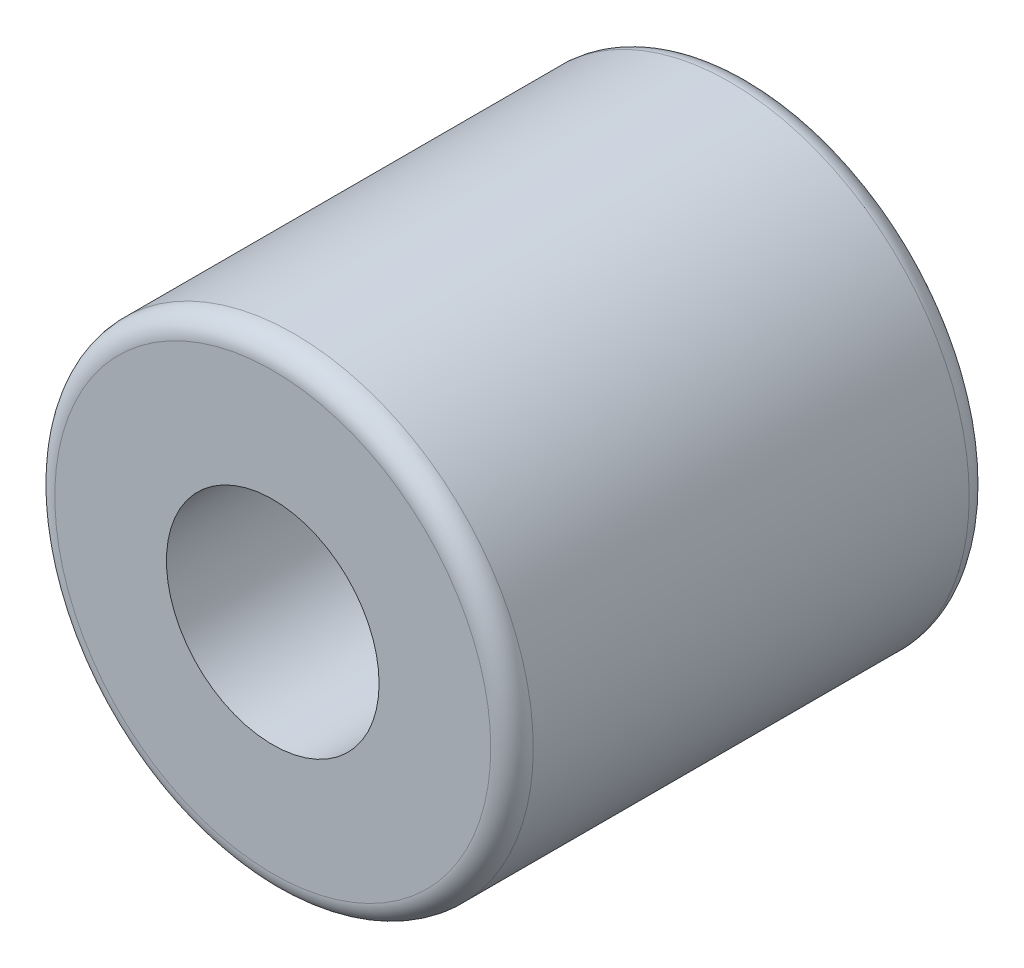
from build123d import *

# Parameters (mm, degrees)
SKETCH_1_R          = 22.5
EXTRUDE_1_DEPTH     = 45
FILLET_1_R          = 2
SKETCH_2_R          = 10
CUT_EXTRUDE_1_DEPTH = 56.113519253


with BuildPart() as part:
    # 草图1 → 凸台-拉伸1 (new body)
    with BuildSketch(Plane.XY):
        with Locations(Location((0, 0, 0), (0, 0, 180))):
            Circle(SKETCH_1_R)
    extrude(amount=EXTRUDE_1_DEPTH)

    # 圆角1
    fillet_1_edges = [part.edges().sort_by_distance(p)[0] for p in [
        (22.5, 0, 0),
        (22.5, 0, 45),
    ]]
    fillet(fillet_1_edges, radius=FILLET_1_R)

    # 草图2 → 切除-拉伸1 (cut, through all)
    with BuildSketch(Plane.XY.offset(45)):
        Circle(SKETCH_2_R)
    extrude(amount=-CUT_EXTRUDE_1_DEPTH, mode=Mode.SUBTRACT)


solid = part.part
